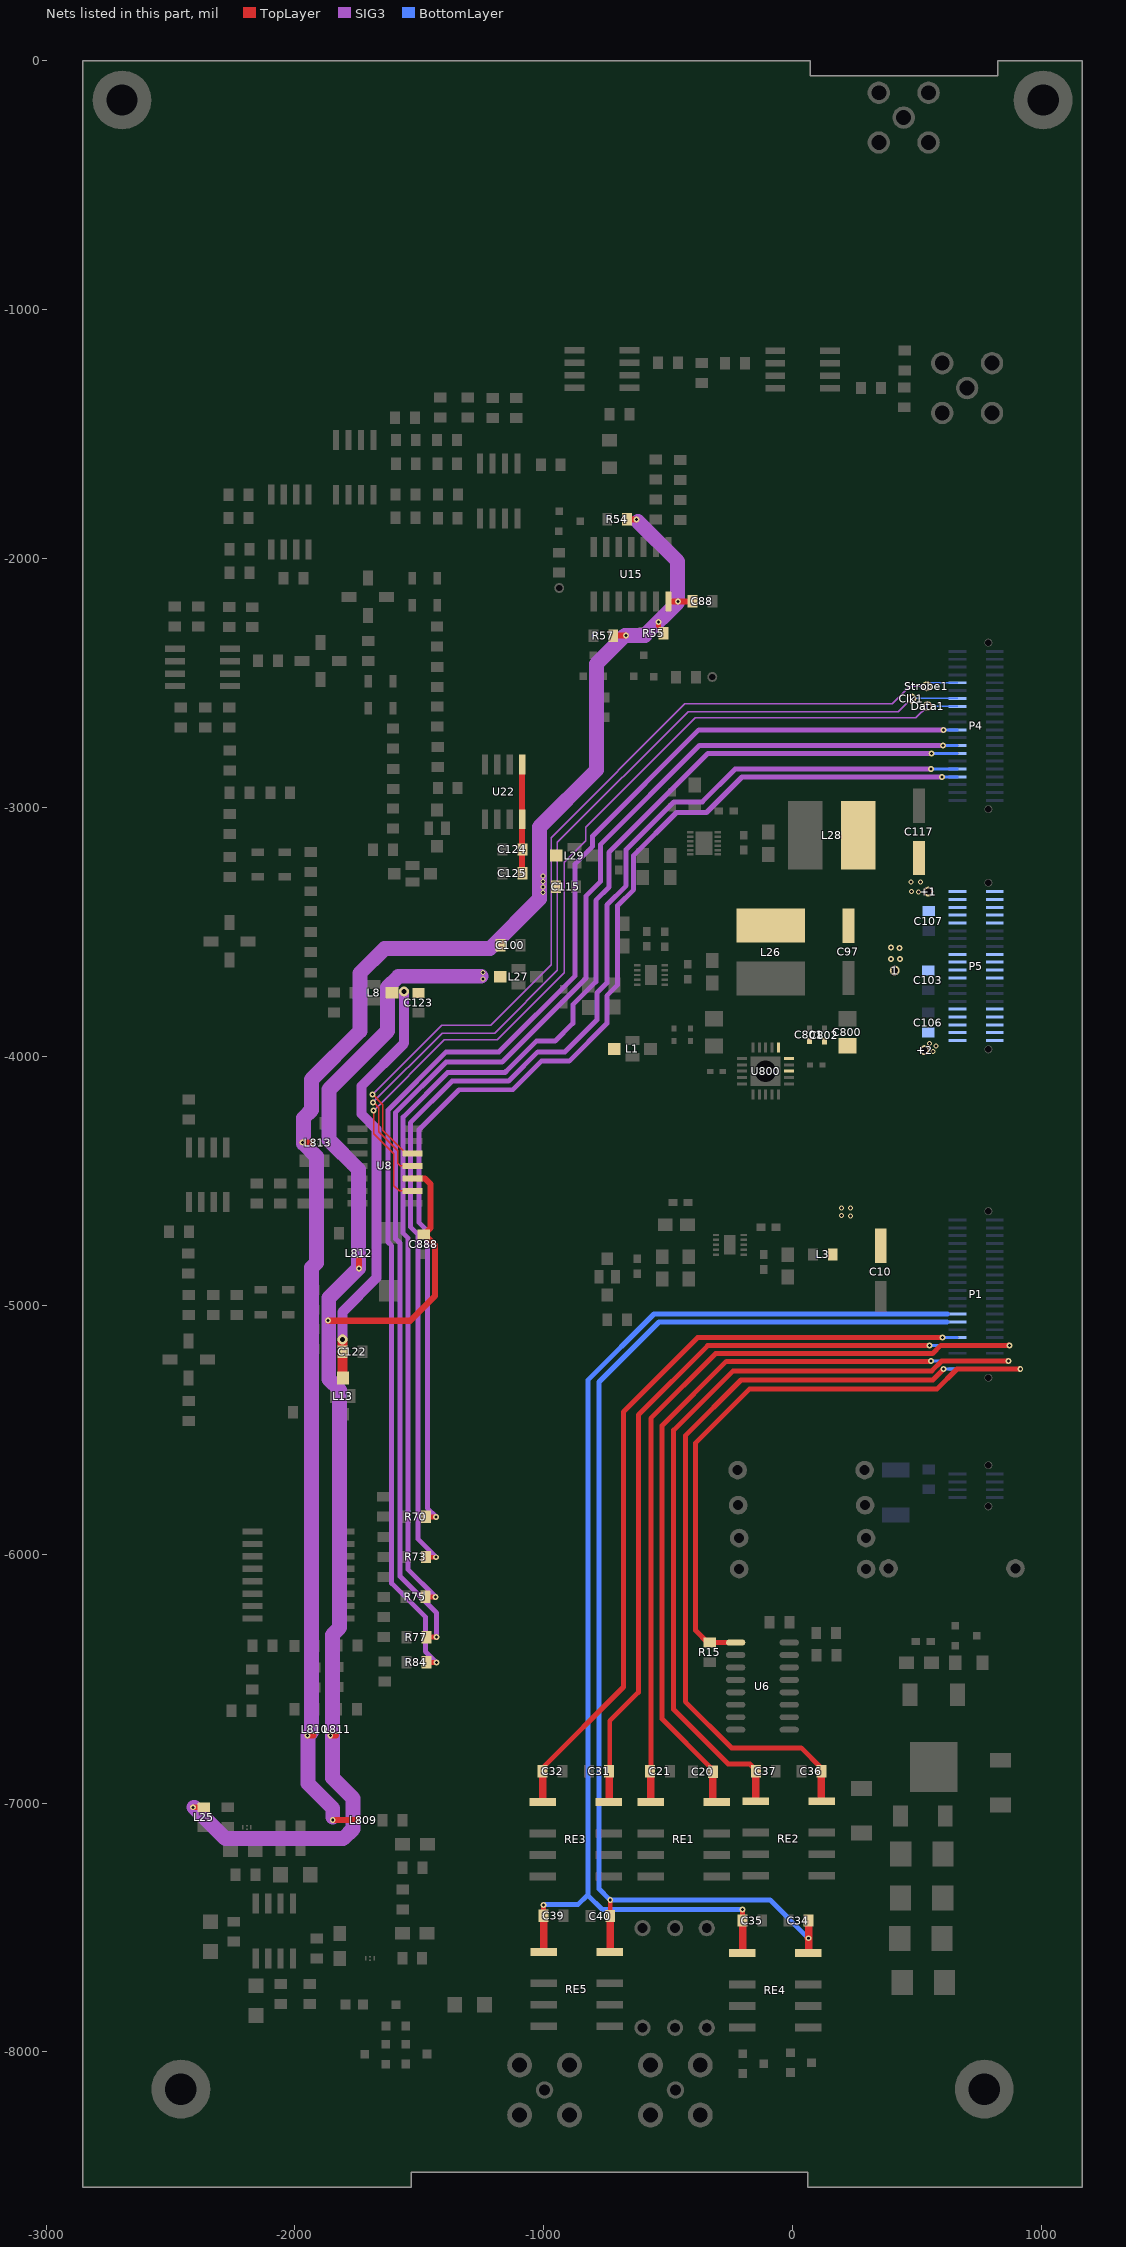
[diagram p0: the nets of this part, all layers, seen from the top]
# Altium PCB MISC109560.PcbDoc (part 2 of 7)
Units mil, origin at the board's own origin, x right, y up, seen from the top; angles counter-clockwise.
Board outline 4015.75 x 8543.31 mil, 4 copper layers (TopLayer, GND, SIG3, BottomLayer); 280 components, 173 nets, 936 pads, 3695 vias.

## Part data
1 +1 +2 Clk1 Data1 HP1 LP1 Strobe1: library part TP
C4 C5 C6 C9 C11 C13 C14 C15 C16 C17 C18 C20 C21 C31 C32 C34 C35 C36 C37 C39 C40 C41 C42 C43 C44 C45 C46 C47 C48 C50 C51 C52 C53 C54 C55 C56 C57 C58 C59 C60 C61 C62 C63 C64 C65 C66 C67 C68 C69 C72 C73 C74 C75 C76 C77 C78 C79 C80 C81 C82 C83 C84 C85 C87 C88 C89 C90 C95 C96 C98 C100 C101 C102 C103 C104 C105 C106 C107 C109 C112 C113 C115 C116 C118 C119 C122 C123 C124 C125 C128 C129 C130 C800 C801 C802 C803 C804 C805 C806 C809 C888: library part CAP, "Capacitor"
C7 C8 C12 C93 C94 C99 C110 C111 C114: library part C1206
C10 C97 C117: library part CAPACITOR_1, "Capacitor"
C49: library part TAJC226K025RNJ
C70 C71 C86: library part "CAPACITOR POL", "Capacitor"
D1 D8 D9 D10 D11 D12: library part BAV99
D2 D3 D4 D5: library part DIODE, "Diode"
J1 J2: library part SMA-KWE
L2 L3 L5 L10 L11 L12 L15 L16 L17 L18 L20 L21 L22 L25 L31 L32: library part INDUCTOR
L26 L28: library part 4.7uH/5a
P1 P4 P5: "Header, 20-Pin, Dual row"
P2: "Header, 4-Pin, Dual row"
P3 P6: library part JA1
Q1: library part NPN, "NPN Transistor"
Q2 Q3 Q4: library part PNP, "PNP Transistor"
R1 R6 R7 R8 R9 R10 R11 R13 R14 R15 R16 R17 R20 R23 R27 R28 R29 R30 R31 R32 R33 R34 R35 R36 R37 R38 R39 R40 R41 R42 R43 R44 R45 R46 R47 R48 R49 R50 R51 R52 R53 R54 R55 R56 R57 R58 R59 R60 R61 R62 R63 R64 R65 R66 R67 R68 R69 R70 R71 R72 R73 R74 R75 R77 R80 R81 R82 R83 R84: library part RES1
R800: library part RES
RE1 RE2 RE3 RE4 RE5: library part AGQ210A4HZ
U15: library part 74HC04
U16: library part AT-250
U17 U20: library part MAR-3SM
U18 U19: library part MAR-6SM
U21: library part MAX4107ESA
U800: library part TPS7A4701RGWR(QFN20)

## Free pads (board coordinates)
  round 236.22 hole 125.98: 0(-2458.3,-8149.61) 0(770.05,-8149.61) 2(1006.27,-157.48) 3(-2694.52,-157.48)

## Via types
v1: diameter 24, hole 12, TopLayer to BottomLayer, 3659 vias
v2: diameter 20, hole 12, TopLayer to BottomLayer, 32 vias
v3: diameter 40, hole 20, TopLayer to BottomLayer, 4 vias

## Nets (pads, with @x,y where several pads share a name; then routed paths per layer and width w, separated by ;. In a path a pad name is that pad's centre, name@x,y a point inside that pad or via, vN(x,y) a via of type N, cw(c..) or ccw(c..) an arc to the next point about the centre after c; other vN are vias at no path point)
+5V: C100.1 C888.1 L25.1 L27.3 L811.3 L812.3 U8.3 | length 5899.4
  TopLayer w10: -1844,-6722 L811.3@-1829,-6722
  TopLayer w24: v1(-2410,-7017) L25.1@-2366,-7017 ; v1(-1858,-6729) -1835,-6729 ; v1(-1742.69,-4852.96) -1742.69,-4817
  TopLayer w25: v1(-1867,-5062) -1537,-5062 -1437,-4962 -1437,-4759 -1481,-4715 C888.1@-1483,-4715 ; U8.3@-1528.37,-4490.35 -1478.65,-4490.35 -1455,-4514 -1455,-4689 C888.1@-1479,-4713
  SIG3 w40: v1@-2408,-7018 -2404,-7018 v1@-2399,-7018
  SIG3 w60: v1@-2405,-7017 -2404,-7018 -2279,-7143 -1806,-7143 -1767,-7104 -1767,-6981 -1849,-6899 -1849,-6324 -1820,-6295 -1820,-5340 -1864,-5296 -1864,-4971 -1745,-4852 -1745,-4454 -1863,-4336 -1863,-4133 -1628,-3898 -1628,-3723 -1583,-3678 -1252,-3678
  other v2: -1244,-3689 -1244,-3663
+12.5V: +2.1 C106.1 C800.1 C801.1 C802.1 P5.31 P5.32 P5.33 P5.34 P5.35 P5.36 P5.37 P5.38 P5.39 P5.40 U800.13 U800.15 U800.16
  other v2: 563,-3980 575,-3958 550,-3949
+12V: C122.1 C123.1 C124.2 C125.2 L1.3 L8.1 L13.1 U22.1 U22.8 | length 2175.3
  TopLayer w24: C125.2@-1086.69,-3259.31 U22.8@-1086.69,-3047 U22.1@-1086.69,-2827
  TopLayer w40: L13.1@-1808,-5284 -1808,-5237 ; C122.1@-1808,-5189 -1808,-5237 ; v3(-1808,-5138) -1808,-5237
  SIG3 w40: v3(-1808,-5138) -1808,-5026 -1673,-4891 -1673,-4292 -1733,-4232 -1733,-4119 -1561,-3947 v3@-1561,-3741
  other v3: -1561,-3740
-5.4V: +1.1 C107.1 C117.2 L28.2 P5.1 P5.2 P5.3 P5.4 P5.5 P5.6 P5.7 P5.8 P5.9 P5.10
  other v2: 505,-3339 478,-3338 476,-3300 514,-3299
-5V: C88.2 C115.2 L29.3 L809.1 L810.3 L813.3 R54.1 R55.2 R57.1 U15.7 | length 6638
  TopLayer w10: -1934,-6722 L810.3@-1921,-6722
  TopLayer w20: -540,-2271.31 v1(-540,-2255.31) ; R55.2@-519,-2299.31 R55.2@-519,-2292.31
  TopLayer w24: v1@-1970,-4345 -1934,-4345 ; v1(-1950,-6729) -1925,-6729 ; v1(-1848,-7069) -1752,-7069
  TopLayer w25: R57.1@-721,-2309.31 v1(-670,-2309.31) ; R54.1@-665,-1842.31 v1(-627,-1842.31) ; U15.7@-492,-2172.31 v1(-460,-2172.31) C88.2@-410,-2172.31
  SIG3 w40: v1(-627,-1842.31) v1@-620.15,-1849.15
  SIG3 w60: -1848,-7056 -1848,-7021 -1947,-6922 -1947,-6729 -1933,-6715 -1933,-4849 -1913.96,-4829.96 -1913.96,-4402.04 -1965,-4351 -1965,-4247 -1933,-4215 -1933,-4093 -1739,-3899 -1739,-3666 -1640,-3567 -1217,-3567 -1017,-3367 -1017,-3078 -789,-2850 -789,-2423 -674,-2308 -594,-2308 -462,-2176 -462,-2011 v1@-622,-1851
  other v1: -1969.96,-4345.31
  other v2: -1003,-3341 -1003,-3319 -1003,-3298 -1003,-3276
A6V: 1.1 C10.1 C97.1 C103.2 L3.1 L26.2 P5.17 P5.18 P5.19 P5.20 P5.21 P5.22 P5.23 P5.24
  other v1: 396,-3608.31 431,-3608.31 430,-3564.31 396,-3563.31
  other v2: 233,-4641 197,-4640 196,-4609 232,-4609
AK2: C21.2 P1.33 RE1.1 | length 3174.5
  TopLayer w20: C21.2@-570,-6870 -570,-5454 -310.31,-5194.31 562,-5194.31 595,-5161.31 831,-5161.31 ; 842.94,-5161.31 831,-5161.31 ; v1@868,-5160.31 867,-5161.31 831,-5161.31
  TopLayer w30: RE1.1@-571,-6986.59 C21.2@-571,-6858.59
  BottomLayer w12: P1.33@812.04,-5161.24 v1(870.94,-5161.24)
AK3: C20.2 P1.38 RE1.8 | length 2868.5
  TopLayer w20: C20.2@-327,-6860 -525,-6662 -525,-5484 -266.31,-5225.31 v1@551,-5225.31 ; C20.2@-321,-6873.59 C20.2@-321,-6861.59
  TopLayer w30: -322,-6978.59 C20.2@-322,-6870.59
  BottomLayer w12: v1(555.07,-5224.24) P1.38@662.43,-5224.24
AK4: C37.1 P1.37 RE2.1 | length 3219.6
  TopLayer w20: C37.1@-151,-6872.59 C37.1@-150,-6872.59 ; C37.1@-148,-6872.59 C37.1@-150,-6872.59 ; C37.1@-146,-6874.59 -148,-6874.59 C37.1@-150,-6872.59 ; C37.1@-145,-6870 -172,-6843 -259,-6843 -478,-6624 -478,-5502 -239.31,-5263.31 559,-5263.31 598,-5224.31 813,-5224.31 ; 839.93,-5224.31 813,-5224.31 ; v1@865,-5224.31 813,-5224.31
  TopLayer w30: RE2.1@-148,-6986.59 -148,-6874.59 C37.1@-148,-6872.59
  BottomLayer w12: P1.37@812.04,-5224.24 v1(867.93,-5224.24)
AK5: C36.1 P1.40 RE2.8 | length 3049.3
  TopLayer w20: C36.1@113,-6859.59 115,-6859.59 C36.1@115,-6872.59 ; C36.1@113,-6857 34,-6778 -246,-6778 -431,-6593 -431,-5524 -207.31,-5300.31 563,-5300.31 v1@605,-5258.31
  TopLayer w30: RE2.8@115,-6982.59 C36.1@115,-6872.59
  BottomLayer w12: v1(606.57,-5255.73) P1.40@662.43,-5255.73
AK6: C31.2 P1.34 RE3.8 | length 2986.9
  TopLayer w20: C31.2@-735,-6882 -735,-6670 -620,-6555 -620,-5441 -341.31,-5162.31 v1(549,-5162.31)
  TopLayer w30: RE3.8@-737.66,-6981.93 C31.2@-737.66,-6882
  BottomLayer w12: v1(549,-5162.31) 553.87,-5162.31 554.94,-5161.24 P1.34@662.43,-5161.24
AK7: C32.2 P1.32 RE3.1 | length 3192.1
  TopLayer w20: C32.2@-1002,-6868 C32.2@-1002.41,-6867.59 ; v1(601.44,-5129.75) -381.75,-5129.75 -680,-5428 -680,-6534 -1004,-6858 -1004,-6866 C32.2@-1002.41,-6867.59 ; C32.2@-1002.41,-6867.59 -1000,-6867.59 C32.2@-1005,-6872.59 -1005,-6867.59 C32.2@-1002.41,-6867.59
  TopLayer w30: RE3.1@-1005,-6983.59 -1005,-6935.59 ; -1005,-6912.59 -1005,-6935.59 ; C32.2@-1005,-6872.59 -1005,-6935.59
  BottomLayer w12: v1(601.44,-5129.75) P1.32@662.43,-5129.75
AK8: C34.2 C40.1 P1.28 RE4.8 RE5.8 | length 4795.1
  TopLayer w20: C40.1@-733,-7445.59 v1(-733,-7389.59)
  TopLayer w30: RE5.8@-732.96,-7595.65 C40.1@-732.96,-7454 ; v1(63,-7543.33) v1@63.74,-7542.59 ; RE4.8@63.74,-7603.95 v1@63.74,-7542.59 ; C34.2@63.74,-7477.59 v1@63.74,-7542.59
  BottomLayer w20: -778,-6921.31 -778,-6910 ; v1@-737,-7386 -778,-7345 -778,-6910 ; v1@-736.8,-7385.8 v1(-733,-7389.59) -90.74,-7389.59 v1(63,-7543.33) ; 621,-5067.31 -537.31,-5067.31 -778,-5308 -778,-6910
AK9: C35.2 C39.1 P1.26 RE4.1 RE5.1 | length 4842.6
  TopLayer w20: C39.1@-1001,-7453.59 v1(-1001,-7409.59) ; C35.2@-202.26,-7472 v1(-202.26,-7427.85)
  TopLayer w30: RE5.1@-1001,-7597.66 C39.1@-1001,-7453.59 ; RE4.1@-201.26,-7603.6 C35.2@-201,-7470.59
  BottomLayer w20: v1@-1000,-7408.59 -863,-7408.59 -824,-7369.59 -823,-7370.59 ; -823,-7371 -823,-7370.59 ; -823,-6947.31 -823,-6934 ; v1(-202.26,-7427.85) -765.74,-7427.85 -823,-7370.59 ; 623,-5035.31 -557.31,-5035.31 -823,-5301 -823,-6934 ; -823,-7370.59 -823,-6934
ATTN1: P4.34 R70.2 | length 4708.6
  TopLayer w20: R70.2@-1473.89,-5850.42 v1(-1432.34,-5850.42)
  SIG3 w20: v1@-1432,-5851 -1468,-5815 -1468,-4701 -1501,-4668 -1501,-4294 -1341,-4134 -1124.69,-4134 -1009.69,-4019 -898,-4019 -747,-3868 -747,-3756.31 -703,-3712.31 -703,-3394 -639,-3330 -639,-3192 -467,-3020 -346,-3020 -203.31,-2877.31 v1@599,-2877.31
  BottomLayer w12: v1(600.46,-2876.76) P4.34@662.43,-2876.76
ATTN2: P4.32 R73.2 | length 4951.3
  TopLayer w20: R73.2@-1473.89,-6012.42 v1(-1432.34,-6012.42)
  SIG3 w20: v1(-1432.34,-6012.42) -1505,-5939.76 -1505,-4716 -1536,-4685 -1536,-4267 -1368,-4099 -1141,-4099 -1132,-4090 ; -1131.85,-4090.15 -1023.69,-3982 -915,-3982 -786.85,-3853.85 -786.85,-3745.15 -746,-3704.31 -746,-3391 -669,-3314 -669,-3169 -477,-2977 -363,-2977 -231.27,-2845.27 v1(555.96,-2845.27) 557.96,-2845.27 v1@558,-2845.31
  BottomLayer w12: v1(555.96,-2845.27) P4.32@662.43,-2845.27
ATTN4: P4.28 R75.2 | length 5174.4
  TopLayer w20: R75.2@-1475.89,-6172.42 v1(-1434.34,-6172.42)
  SIG3 w20: v1(-1434.34,-6172.42) -1546,-6060.76 -1546,-4729 -1565,-4710 -1565,-4244 -1386,-4065 -1156,-4065 -1141,-4050 ; -1140.85,-4050.15 -1029.69,-3939 -955,-3939 -883,-3867 -883,-3792.31 -791,-3700.31 -791,-3373 -738,-3320 -738,-3180 -340.28,-2782.28 v1(558.03,-2782.28)
  BottomLayer w12: v1(558.03,-2782.28) P4.28@662.43,-2782.28
ATTN8: P4.26 R77.2 | length 5366.6
  TopLayer w20: R77.2@-1472.89,-6333.42 v1(-1431.34,-6333.42)
  SIG3 w20: v1(-1431.34,-6333.42) -1431.34,-6235.66 -1578,-6089 -1578,-4750 -1595,-4733 -1595,-4225 -1393,-4023 -1167.69,-4023 -830,-3685.31 -830,-3355 -773,-3298 -773,-3149 -374.78,-2750.78 v1(603.53,-2750.78)
  BottomLayer w12: v1(603.53,-2750.78) P4.26@662.43,-2750.78
ATTN16: P4.22 R84.2 | length 5548.7
  TopLayer w20: R84.2@-1472.89,-6434.42 v1(-1431.34,-6434.42)
  SIG3 w20: -1476,-6292 -1476,-6252 -1611,-6117 -1611,-4761 -1626,-4746 -1626,-4216 -1392,-3982 -1179.69,-3982 -874,-3676.31 -874,-3226.46 -803.5,-3155.96 -803.5,-3114.5 -376.79,-2687.79 v1(605.52,-2687.79) ; -1475.93,-6292 -1475.93,-6391.01 v1@-1433.93,-6433.01 ; v1@-1432.34,-6433.42 v1(-1431.34,-6434.42)
  BottomLayer w12: v1(605.52,-2687.79) P4.22@662.43,-2687.79
"DAC CLK": Clk1.1 P4.14 U8.4 | length 3667.3
  TopLayer w6: v1@-1682,-4187 -1663,-4206 -1663,-4303 -1587,-4379 -1587,-4430 -1576.65,-4440.35 U8.4@-1528.37,-4440.35
  SIG3 w6: v1(-1687,-4185) -1409,-3907 -1198,-3907 -945,-3654 -945,-3140 -420,-2615 424,-2615 Clk1.1@477,-2562
  BottomLayer w6: Clk1.1@477.8,-2561.8 P4.14@662.43,-2561.8
"DAC DATA": Data1.1 P4.16 U8.2 | length 3723
  TopLayer w6: v1@-1683,-4216 -1683,-4310 -1602,-4391 -1602,-4519 -1580.65,-4540.35 U8.2@-1528.37,-4540.35
  SIG3 w6: v1(-1684,-4218) -1400,-3934 -1187,-3934 -917,-3664 -917,-3219 -831,-3133 -831,-3080 -391,-2640 495,-2640 Data1.1@542,-2593
  BottomLayer w6: Data1.1@549.3,-2593.3 P4.16@662.43,-2593.3
"DAC STROBE": P4.10 Strobe1.1 U8.5 | length 3623.6
  TopLayer w6: v1(-1688,-4153) -1647,-4194 -1647,-4296 -1552.65,-4390.35 U8.5@-1528.37,-4390.35
  SIG3 w6: v1(-1688,-4153) -1410,-3875 -1213,-3875 -970,-3632 -970,-3121 -433,-2584 400,-2584 471,-2513 Strobe1.1@531,-2513
  BottomLayer w6: 554.19,-2498.81 P4.10@662.43,-2498.81
DATA_T: P1.39 R15.2 U6.1 | length 2576.6
  TopLayer w20: R15.2@-342,-6355 -390,-6307 -390,-5553 -174.31,-5337.31 579,-5337.31 660,-5256.31 762,-5256.31 ; R15.2@-333,-6355.31 U6.1@-229,-6355.31 ; 886.43,-5256.31 762,-5256.31 ; v1@911,-5256.31 762,-5256.31
  BottomLayer w12: P1.39@812.04,-5255.73 v1(914.43,-5255.73)